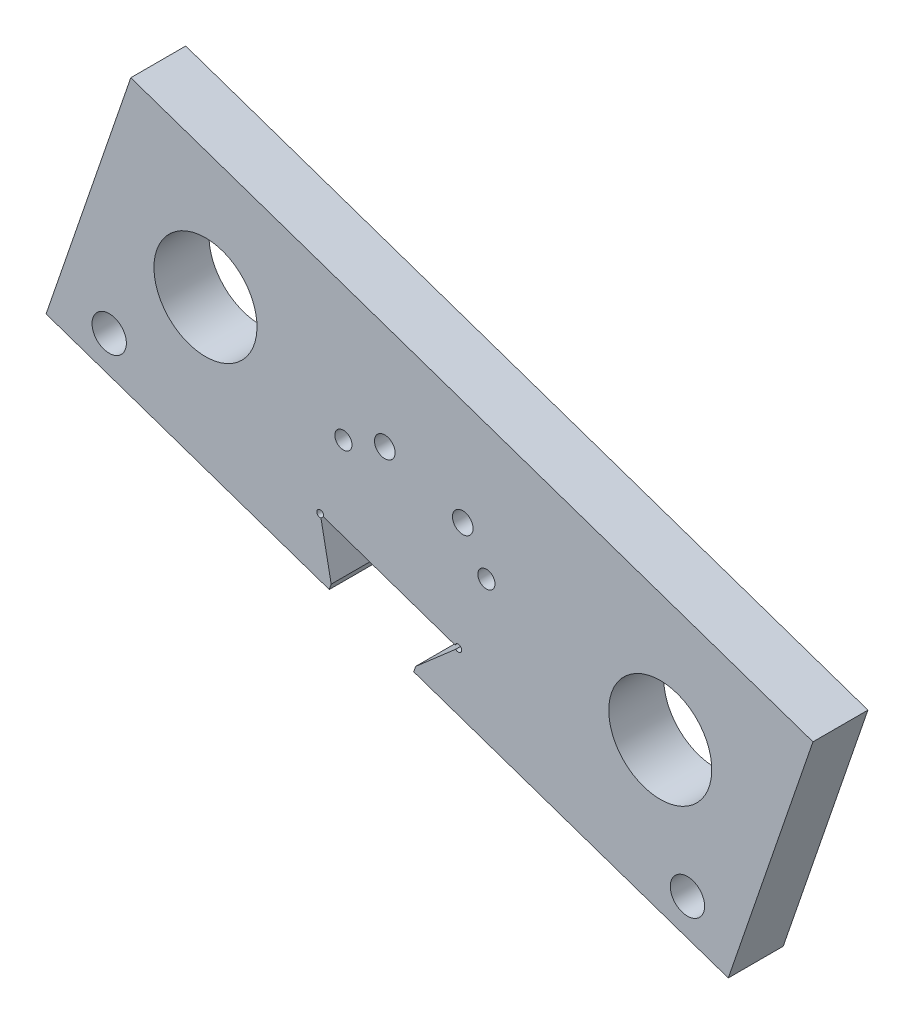
from build123d import *

# Parameters (mm, degrees)
SKETCH_1_R             = 7.5
EXTRUDE_1_DEPTH        = 8
SKETCH_2_W             = 105
SKETCH_2_H             = 8
EXTRUDE_2_DEPTH        = 3
CUT_EXTRUDE_1_DEPTH    = 326.744737494
HOLE_WIZARD_M6_1_D     = 5
HOLE_WIZARD_M6_1_DEPTH = 15
HOLE_WIZARD_M6_1_TIP   = 1.502151548
HOLE_WIZARD_M3_1_D     = 2.5
MM_1_D                 = 3
CUT_EXTRUDE_2_DEPTH    = 10
SKETCH_14_R            = 0.5
CUT_EXTRUDE_3_DEPTH    = 326.744737494


with BuildPart() as part:
    # 草图1 → 凸台-拉伸1 (new body)
    with BuildSketch(Plane.XY):
        Polygon((-123.272913695, 191.443187885), (-134.630416513, 158.337189489), (-233.948411698, 192.409697944), (-222.59090888, 225.515696339), align=None)
        with Locations(Location((-211.716661092, 203.283945733, 0), (0, 0, 90))):
            Circle(SKETCH_1_R, mode=Mode.SUBTRACT)
        with Locations(Location((-145.504664302, 180.568940096, 0), (0, 0, 90))):
            Circle(SKETCH_1_R, mode=Mode.SUBTRACT)
    extrude(amount=EXTRUDE_1_DEPTH)

    # 草图2 → 凸台-拉伸2 (add)
    with BuildSketch(Plane(origin=(34.423389522, 100.340778821, 0), x_dir=(0.9458856684293921, -0.3245000805236912, 0), z_dir=(-0.3245000805236912, -0.9458856684293921, 0))):
        with Locations((-231.225412254, 4)):
            Rectangle(SKETCH_2_W, SKETCH_2_H)
    extrude(amount=EXTRUDE_2_DEPTH)

    # 草图3 → 切除-拉伸1 (cut, through all)
    with BuildSketch(Plane.XY.offset(8)):
        Polygon((-181.873786677, 171.373096295), (-193.224414699, 175.267097261), (-194.997272817, 184.33298428), (-174.908927271, 177.441379972), align=None)
    extrude(amount=-CUT_EXTRUDE_1_DEPTH, mode=Mode.SUBTRACT)

    # M6 螺纹孔1
    with Locations(Plane.XY.offset(8)):
        with Locations((-141.5485017, 162.824961471), (-225.73232619, 191.705468637)):
            Hole(HOLE_WIZARD_M6_1_D / 2, depth=HOLE_WIZARD_M6_1_DEPTH)
            with Locations((0, 0, -(HOLE_WIZARD_M6_1_DEPTH + HOLE_WIZARD_M6_1_TIP / 2))):  # 118° drill point
                Cone(0, HOLE_WIZARD_M6_1_D / 2, HOLE_WIZARD_M6_1_TIP, mode=Mode.SUBTRACT)

    # M3 螺纹孔1 (through all)
    with Locations(Plane(origin=(0, 0, 0), x_dir=(-1, 0, 0), z_dir=(0, 0, -1))):
        with Locations((170.819179959, 188.188267601), (191.635646748, 195.306884773)):
            Hole(HOLE_WIZARD_M3_1_D / 2)

    # 大小mm 暗销孔1 (through all)
    with Locations(Plane(origin=(0, 0, 0), x_dir=(-1, 0, 0), z_dir=(0, 0, -1))):
        with Locations((174.256171582, 193.590156353), (185.610608012, 197.473038447)):
            Hole(MM_1_D / 2)

    # 草图13 → 切除-拉伸2 (cut)
    with BuildSketch(Plane.XY.offset(8)):
        Polygon((-193.697357533, 175.429347302), (-192.732083432, 178.243025921), (-180.825057933, 172.889205286), (-181.400843843, 171.210846255), align=None)
    extrude(amount=-CUT_EXTRUDE_2_DEPTH, mode=Mode.SUBTRACT)

    # 草图14 → 切除-拉伸3 (cut, through all)
    with BuildSketch(Plane.XY.offset(8)):
        with Locations((-194.997272817, 184.33298428)):
            Circle(SKETCH_14_R)
        with Locations((-174.908927271, 177.441379972)):
            Circle(SKETCH_14_R)
    extrude(amount=-CUT_EXTRUDE_3_DEPTH, mode=Mode.SUBTRACT)


solid = part.part
